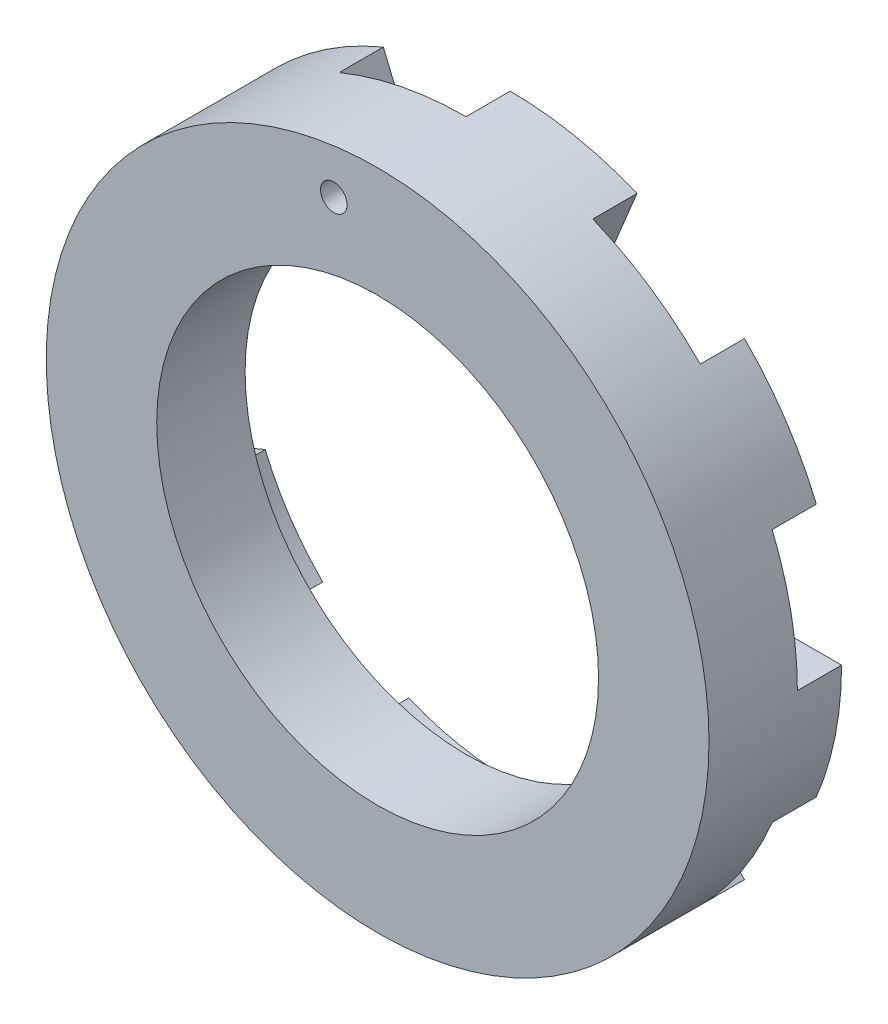
from build123d import *

# Parameters (mm, degrees)
SKETCH1_R           = 37.5
SKETCH1_R_2         = 25
BOSS_EXTRUDE1_DEPTH = 15
SKETCH2_R           = 30
CUT_EXTRUDE1_DEPTH  = 5
CUT_EXTRUDE2_DEPTH  = 5
SKETCH4_R           = 1.5
CUT_EXTRUDE3_DEPTH  = 10


with BuildPart() as part:
    # Sketch1 → Boss-Extrude1 (new body)
    with BuildSketch(Plane.XY):
        Circle(SKETCH1_R)
        Circle(SKETCH1_R_2, mode=Mode.SUBTRACT)
    extrude(amount=BOSS_EXTRUDE1_DEPTH)

    # Sketch2 → Cut-Extrude1 (cut)
    with BuildSketch(Plane(origin=(0, 0, 0), x_dir=(-1, 0, 0), z_dir=(0, 0, -1))):
        Circle(SKETCH2_R)
    extrude(amount=-CUT_EXTRUDE1_DEPTH, mode=Mode.SUBTRACT)

    # Sketch3 → Cut-Extrude2 (cut)
    with BuildSketch(Plane(origin=(0, 0, 0), x_dir=(-1, 0, 0), z_dir=(0, 0, -1))):
        with BuildLine():
            Line((0, 30), (0, 37.5))
            ThreePointArc((0, 37.5), (7.315887076, 36.779448015), (14.350628714, 34.645482469))
            Line((14.350628714, 34.645482469), (11.480502971, 27.716385975))
            ThreePointArc((11.480502971, 27.716385975), (5.85270966, 29.423558412), (0, 30))
        make_face()
        with BuildLine():
            Line((21.213203436, 21.213203436), (26.516504294, 26.516504294))
            ThreePointArc((26.516504294, 26.516504294), (31.180110461, 20.833883738), (34.645482469, 14.350628714))
            Line((34.645482469, 14.350628714), (27.716385975, 11.480502971))
            ThreePointArc((27.716385975, 11.480502971), (24.944088369, 16.667106991), (21.213203436, 21.213203436))
        make_face()
        with BuildLine():
            Line((30, 0), (37.5, 0))
            ThreePointArc((37.5, 0), (36.779448015, -7.315887076), (34.645482469, -14.350628714))
            Line((34.645482469, -14.350628714), (27.716385975, -11.480502971))
            ThreePointArc((27.716385975, -11.480502971), (29.423558412, -5.85270966), (30, 0))
        make_face()
        with BuildLine():
            Line((21.213203436, -21.213203436), (26.516504294, -26.516504294))
            ThreePointArc((26.516504294, -26.516504294), (20.833883738, -31.180110461), (14.350628714, -34.645482469))
            Line((14.350628714, -34.645482469), (11.480502971, -27.716385975))
            ThreePointArc((11.480502971, -27.716385975), (16.667106991, -24.944088369), (21.213203436, -21.213203436))
        make_face()
        with BuildLine():
            Line((0, -30), (0, -37.5))
            ThreePointArc((0, -37.5), (-7.315887076, -36.779448015), (-14.350628714, -34.645482469))
            Line((-14.350628714, -34.645482469), (-11.480502971, -27.716385975))
            ThreePointArc((-11.480502971, -27.716385975), (-5.85270966, -29.423558412), (0, -30))
        make_face()
        with BuildLine():
            Line((-21.213203436, -21.213203436), (-26.516504294, -26.516504294))
            ThreePointArc((-26.516504294, -26.516504294), (-31.180110461, -20.833883738), (-34.645482469, -14.350628714))
            Line((-34.645482469, -14.350628714), (-27.716385975, -11.480502971))
            ThreePointArc((-27.716385975, -11.480502971), (-24.944088369, -16.667106991), (-21.213203436, -21.213203436))
        make_face()
        with BuildLine():
            Line((-30, 0), (-37.5, 0))
            ThreePointArc((-37.5, 0), (-36.779448015, 7.315887076), (-34.645482469, 14.350628714))
            Line((-34.645482469, 14.350628714), (-27.716385975, 11.480502971))
            ThreePointArc((-27.716385975, 11.480502971), (-29.423558412, 5.85270966), (-30, 0))
        make_face()
        with BuildLine():
            Line((-21.213203436, 21.213203436), (-26.516504294, 26.516504294))
            ThreePointArc((-26.516504294, 26.516504294), (-20.833883738, 31.180110461), (-14.350628714, 34.645482469))
            Line((-14.350628714, 34.645482469), (-11.480502971, 27.716385975))
            ThreePointArc((-11.480502971, 27.716385975), (-16.667106991, 24.944088369), (-21.213203436, 21.213203436))
        make_face()
    extrude(amount=-CUT_EXTRUDE2_DEPTH, mode=Mode.SUBTRACT)

    # Sketch4 → Cut-Extrude3 (cut)
    with BuildSketch(Plane(origin=(0, 0, 5), x_dir=(-1, 0, 0), z_dir=(0, 0, -1))):
        with Locations((4.960455731, 32.119213548)):
            Circle(SKETCH4_R)
    extrude(amount=-CUT_EXTRUDE3_DEPTH, mode=Mode.SUBTRACT)


solid = part.part
